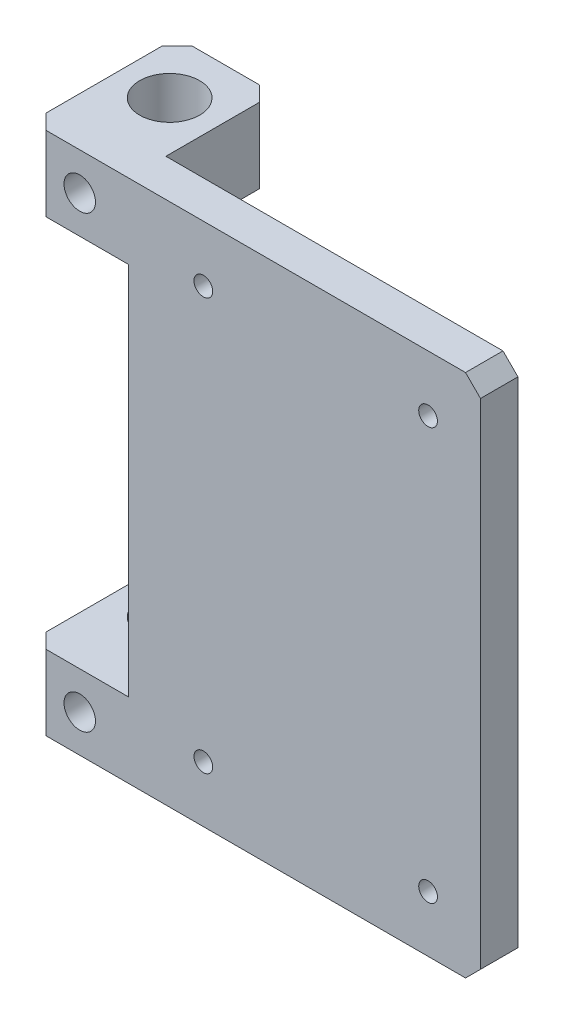
from build123d import *

# Parameters (mm, degrees)
BOSS_EXTRUDE1_DEPTH   = 70
SKETCH2_R             = 0.75
CUT_EXTRUDE1_DEPTH    = 10
SKETCH3_W             = 25
SKETCH3_H             = 50
CUT_EXTRUDE2_DEPTH    = 13
SKETCH4_R             = 4
CUT_EXTRUDE3_DEPTH    = 96.524865873
SKETCH5_W             = 13
SKETCH5_H             = 50
BOSS_EXTRUDE2_DEPTH   = 5
SKETCH9_W             = 13
SKETCH9_H             = 5.5
CUT_EXTRUDE6_DEPTH    = 71
LPATTERN1_COUNT       = 2
LPATTERN1_PITCH       = 30
SKETCH10_W            = 13
SKETCH10_H            = 50
CUT_EXTRUDE7_DEPTH    = 95.235078394
CHAMFER1_SIZE         = 2
CHAMFER2_SIZE         = 2
M3_TAPPED_HOLE1_D     = 2.5
M3_TAPPED_HOLE1_DEPTH = 7.5
M3_TAPPED_HOLE1_TIP   = 0.751075774
M5_TAPPED_HOLE1_D     = 4.2
M5_TAPPED_HOLE1_DEPTH = 12.4
M5_TAPPED_HOLE1_TIP   = 1.2618073
M5_TAPPED_HOLE2_D     = 4.2
M5_TAPPED_HOLE2_DEPTH = 12.4
M5_TAPPED_HOLE2_TIP   = 1.2618073
CHAMFER3_SIZE         = 0.8


with BuildPart() as part:
    # Sketch1 → Boss-Extrude1 (new body)
    with BuildSketch(Plane(origin=(0, 0, 0), x_dir=(1, 0, 0), z_dir=(0, 1, 0))):
        Polygon((0, 0), (60, 0), (60, 5), (13, 5), (13, 25), (0, 25), align=None)
    extrude(amount=BOSS_EXTRUDE1_DEPTH)

    # Sketch2 → Cut-Extrude1 (cut)
    with BuildSketch(Plane.XY):
        with Locations((53, 62.5)):
            Circle(SKETCH2_R)
        with Locations((53, 7.5)):
            Circle(SKETCH2_R)
    cut_extrude1 = extrude(amount=-CUT_EXTRUDE1_DEPTH, mode=Mode.SUBTRACT)

    # Sketch3 → Cut-Extrude2 (cut)
    with BuildSketch(Plane.ZY):
        with Locations((-12.5, 35)):
            Rectangle(SKETCH3_W, SKETCH3_H)
    extrude(amount=-CUT_EXTRUDE2_DEPTH, mode=Mode.SUBTRACT)

    # Sketch4 → Cut-Extrude3 (cut, through all)
    with BuildSketch(Plane(origin=(0, 70, 0), x_dir=(1, 0, 0), z_dir=(0, 1, 0))):
        with Locations(Location((6.5, 12, 0), (0, 0, 270))):
            Circle(SKETCH4_R)
    extrude(amount=-CUT_EXTRUDE3_DEPTH, mode=Mode.SUBTRACT)

    # Sketch5 → Boss-Extrude2 (add)
    with BuildSketch(Plane.XY):
        with Locations((6.5, 35)):
            Rectangle(SKETCH5_W, SKETCH5_H)
    extrude(amount=-BOSS_EXTRUDE2_DEPTH)

    # Sketch9 → Cut-Extrude6 (cut)
    with BuildSketch(Plane(origin=(0, 70, 0), x_dir=(1, 0, 0), z_dir=(0, 1, 0))):
        with Locations((6.5, 22.25)):
            Rectangle(SKETCH9_W, SKETCH9_H)
    extrude(amount=-CUT_EXTRUDE6_DEPTH, mode=Mode.SUBTRACT)

    # LPattern1: Cut-Extrude1 ×2
    with Locations(*[(-i * LPATTERN1_PITCH, 0, 0) for i in range(1, LPATTERN1_COUNT)]):
        add(cut_extrude1, mode=Mode.SUBTRACT)

    # Sketch10 → Cut-Extrude7 (cut, through all)
    with BuildSketch(Plane(origin=(0, 0, -19.5), x_dir=(-1, 0, 0), z_dir=(0, 0, -1))):
        with Locations((-6.5, 35)):
            Rectangle(SKETCH10_W, SKETCH10_H)
    extrude(amount=-CUT_EXTRUDE7_DEPTH, mode=Mode.SUBTRACT)

    # Chamfer1
    chamfer1_edges = [part.edges().sort_by_distance(p)[0] for p in [
        (0, 65, 0),
        (0, 5, 0),
        (0, 5, -19.5),
        (0, 65, -19.5),
        (13, 5, -19.5),
        (13, 65, -19.5),
    ]]
    chamfer(chamfer1_edges, length=CHAMFER1_SIZE)

    # Chamfer2
    chamfer2_edges = [part.edges().sort_by_distance(p)[0] for p in [
        (60, 70, -2.5),
        (60, 0, -2.5),
    ]]
    chamfer(chamfer2_edges, length=CHAMFER2_SIZE)

    # M3 Tapped Hole1
    with Locations(Plane(origin=(23, 7.5, -5), x_dir=(-1, 0, 0), z_dir=(0, 0, -1))):
        with Locations((0, 0), (-30, 0), (-30, 55), (0, 55)):
            Hole(M3_TAPPED_HOLE1_D / 2, depth=M3_TAPPED_HOLE1_DEPTH)
            with Locations((0, 0, -(M3_TAPPED_HOLE1_DEPTH + M3_TAPPED_HOLE1_TIP / 2))):  # 118° drill point
                Cone(0, M3_TAPPED_HOLE1_D / 2, M3_TAPPED_HOLE1_TIP, mode=Mode.SUBTRACT)

    # M5 Tapped Hole1
    with Locations(Plane(origin=(6.5, 5, 0), x_dir=(1, 0, 0), z_dir=(0, 0, 1))):
        with Locations((0, 0)):
            Hole(M5_TAPPED_HOLE1_D / 2, depth=M5_TAPPED_HOLE1_DEPTH)
            with Locations((0, 0, -(M5_TAPPED_HOLE1_DEPTH + M5_TAPPED_HOLE1_TIP / 2))):  # 118° drill point
                Cone(0, M5_TAPPED_HOLE1_D / 2, M5_TAPPED_HOLE1_TIP, mode=Mode.SUBTRACT)

    # M5 Tapped Hole2
    with Locations(Plane(origin=(6.5, 65, 0), x_dir=(1, 0, 0), z_dir=(0, 0, 1))):
        with Locations((0, 0)):
            Hole(M5_TAPPED_HOLE2_D / 2, depth=M5_TAPPED_HOLE2_DEPTH)
            with Locations((0, 0, -(M5_TAPPED_HOLE2_DEPTH + M5_TAPPED_HOLE2_TIP / 2))):  # 118° drill point
                Cone(0, M5_TAPPED_HOLE2_D / 2, M5_TAPPED_HOLE2_TIP, mode=Mode.SUBTRACT)

    # Chamfer3
    chamfer3_edges = [part.edges().sort_by_distance(p)[0] for p in [
        (21.75, 62.5, -5),
        (51.75, 62.5, -5),
        (51.75, 7.5, -5),
        (21.75, 7.5, -5),
    ]]
    chamfer(chamfer3_edges, length=CHAMFER3_SIZE)


solid = part.part
